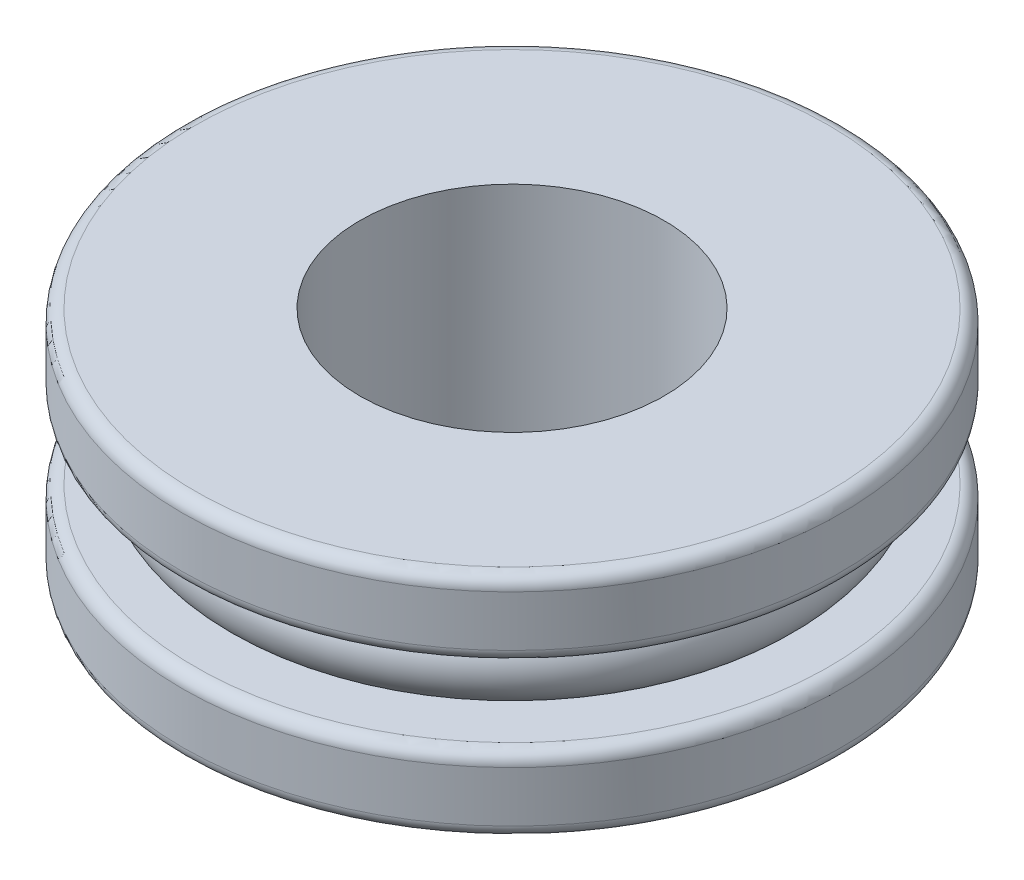
SolidWorks part; units mm, degrees
ref_plane "Front Plane" through (0, 0, 0) normal (0, 0, 1) x (1, 0, 0)
ref_plane "Top Plane" through (0, 0, 0) normal (0, 1, 0) x (1, 0, 0)
ref_plane "Right Plane" through (0, 0, 0) normal (1, 0, 0) x (0, 0, -1)
sketch "Sketch1" plane through (0, 0, 0) normal (0, 0, 1) x (1, 0, 0)
  line L0 (6, 0) -> (13, 0)
  line L1 (13, 0) -> (13, -3)
  line L2 (13, -3) -> (10, -3)
  line L3 (10, -6) -> (13, -6)
  line L4 (13, -6) -> (13, -9)
  line L5 (13, -9) -> (6, -9)
  line L6 (6, 0) -> (6, -9)
  line L7 (0, 0) -> (0, -34.3636) construction
  arc A0 (10, -3) -> (10, -6) centre (10, -4.5) cw
  dimension "D3" = 1.5
  dimension "D7" = 4
  dimension "D1" = 9
  dimension "D2" = 3
  dimension "D4" = 12
  dimension "D5" = 26
  dimension "D6" = 0
revolve "Revolve1" add sketch "Sketch1" angle 360 about L7
fillet "Fillet1" radius 0.5 4 edges at (0, -9, 13) (0, -6, 13) (0, 0, 13) (0, -3, 13)
